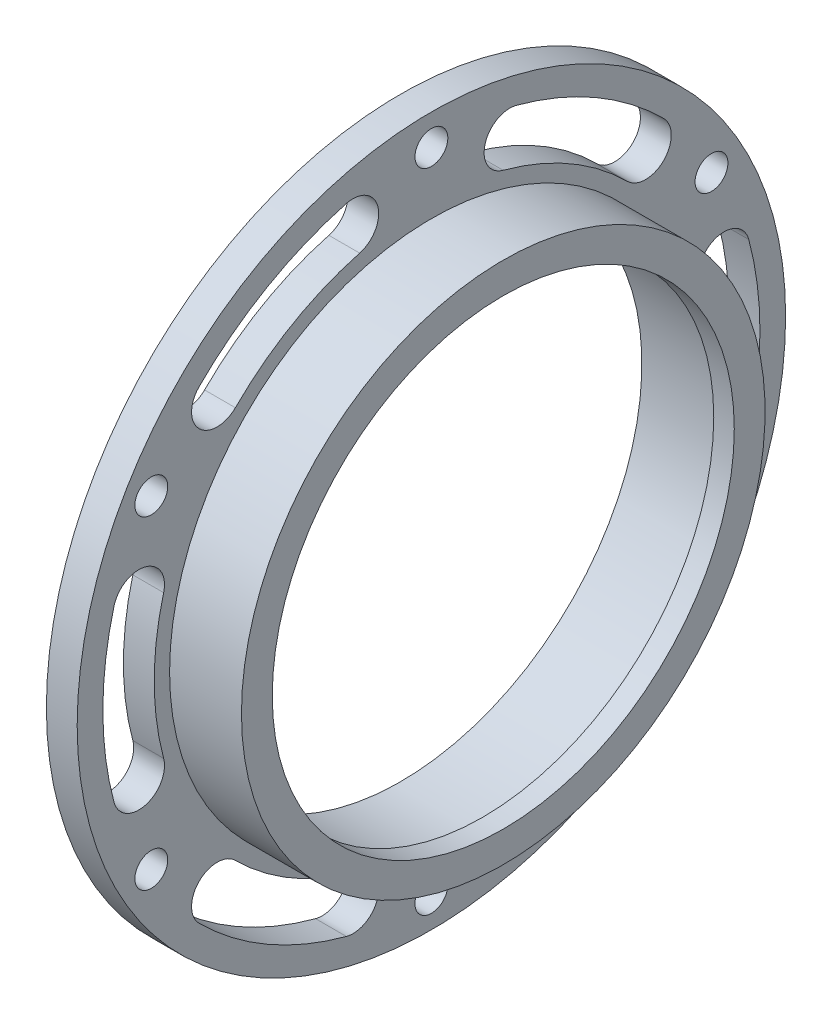
from build123d import *

# Parameters (mm, degrees)
SKETCH_2_R          = 1.6
CUT_EXTRUDE_1_DEPTH = 50.289958409
CUT_EXTRUDE_2_DEPTH = 50.289958409


with BuildPart() as part:
    # 草图1 → 旋转1 (revolve)
    with BuildSketch(Plane(origin=(0, 0, 0), x_dir=(1, 0, 0), z_dir=(0, 1, 0)), mode=Mode.PRIVATE) as revolve_1_sk:
        Polygon((0, 23.5), (0, 34.5), (3, 34.5), (3, 25.5), (10, 25.5), (10, 22.5), (8, 22.5), (8, 23.5), align=None)
    revolve(revolve_1_sk.sketch.rotate(Axis((-505.796489034, 0, 0), (1, 0, 0)), 180), axis=Axis((-505.796489034, 0, 0), (1, 0, 0)))

    # 草图2 → 切除-拉伸1 (cut, through all)
    with BuildSketch(Plane(origin=(3, 0, 0), x_dir=(0, 0, -1), z_dir=(1, 0, 0))):
        with Locations((0, 31.5)):
            Circle(SKETCH_2_R)
        with Locations((27.279800219, 15.75)):
            Circle(SKETCH_2_R)
        with Locations((27.279800219, -15.75)):
            Circle(SKETCH_2_R)
        with Locations((0, -31.5)):
            Circle(SKETCH_2_R)
        with Locations((-27.279800219, -15.75)):
            Circle(SKETCH_2_R)
        with Locations((-27.279800219, 15.75)):
            Circle(SKETCH_2_R)
    extrude(amount=-CUT_EXTRUDE_1_DEPTH, mode=Mode.SUBTRACT)

    # 草图3 → 切除-拉伸2 (cut, through all)
    with BuildSketch(Plane(origin=(3, 0, 0), x_dir=(0, 0, -1), z_dir=(1, 0, 0))):
        with BuildLine():
            ThreePointArc((22.627416998, 22.627416998), (16, 27.712812921), (8.282209443, 30.909626441))
            ThreePointArc((8.282209443, 30.909626441), (5.220347265, 29.141859488), (6.988114218, 26.07999731))
            ThreePointArc((6.988114218, 26.07999731), (13.5, 23.382685902), (19.091883092, 19.091883092))
            ThreePointArc((19.091883092, 19.091883092), (22.627416998, 19.091883092), (22.627416998, 22.627416998))
        make_face()
        with BuildLine():
            ThreePointArc((30.909626441, -8.282209443), (32, 0), (30.909626441, 8.282209443))
            ThreePointArc((30.909626441, 8.282209443), (27.847764263, 10.049976396), (26.07999731, 6.988114218))
            ThreePointArc((26.07999731, 6.988114218), (27, 0), (26.07999731, -6.988114218))
            ThreePointArc((26.07999731, -6.988114218), (27.847764263, -10.049976396), (30.909626441, -8.282209443))
        make_face()
        with BuildLine():
            ThreePointArc((8.282209443, -30.909626441), (16, -27.712812921), (22.627416998, -22.627416998))
            ThreePointArc((22.627416998, -22.627416998), (22.627416998, -19.091883092), (19.091883092, -19.091883092))
            ThreePointArc((19.091883092, -19.091883092), (13.5, -23.382685902), (6.988114218, -26.07999731))
            ThreePointArc((6.988114218, -26.07999731), (5.220347265, -29.141859488), (8.282209443, -30.909626441))
        make_face()
        with BuildLine():
            ThreePointArc((-22.627416998, -22.627416998), (-16, -27.712812921), (-8.282209443, -30.909626441))
            ThreePointArc((-8.282209443, -30.909626441), (-5.220347265, -29.141859488), (-6.988114218, -26.07999731))
            ThreePointArc((-6.988114218, -26.07999731), (-13.5, -23.382685902), (-19.091883092, -19.091883092))
            ThreePointArc((-19.091883092, -19.091883092), (-22.627416998, -19.091883092), (-22.627416998, -22.627416998))
        make_face()
        with BuildLine():
            ThreePointArc((-30.909626441, 8.282209443), (-32, 0), (-30.909626441, -8.282209443))
            ThreePointArc((-30.909626441, -8.282209443), (-27.847764263, -10.049976396), (-26.07999731, -6.988114218))
            ThreePointArc((-26.07999731, -6.988114218), (-27, 0), (-26.07999731, 6.988114218))
            ThreePointArc((-26.07999731, 6.988114218), (-27.847764263, 10.049976396), (-30.909626441, 8.282209443))
        make_face()
        with BuildLine():
            ThreePointArc((-8.282209443, 30.909626441), (-16, 27.712812921), (-22.627416998, 22.627416998))
            ThreePointArc((-22.627416998, 22.627416998), (-22.627416998, 19.091883092), (-19.091883092, 19.091883092))
            ThreePointArc((-19.091883092, 19.091883092), (-13.5, 23.382685902), (-6.988114218, 26.07999731))
            ThreePointArc((-6.988114218, 26.07999731), (-5.220347265, 29.141859488), (-8.282209443, 30.909626441))
        make_face()
    extrude(amount=-CUT_EXTRUDE_2_DEPTH, mode=Mode.SUBTRACT)


solid = part.part
